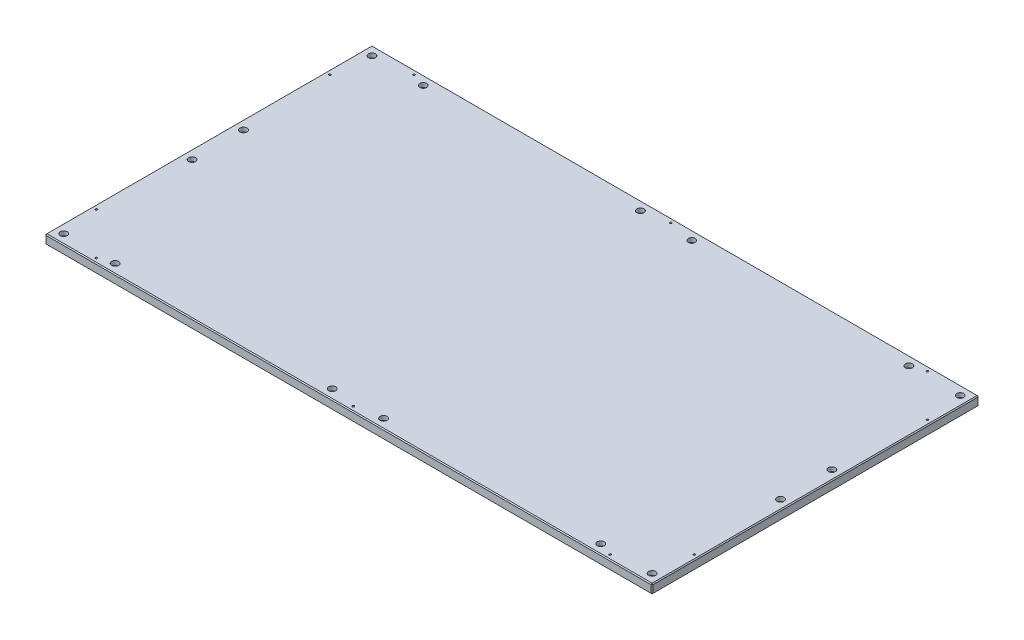
from build123d import *

# Parameters (mm, degrees)
SKETCH_1_W                          = 1300
SKETCH_1_H                          = 700
EXTRUDE_1_DEPTH                     = 10
CHAMFER_1_SIZE                      = 2
HOLE_WIZARD_1_D                     = 9
HOLE_WIZARD_1_CBORE_D               = 15
HOLE_WIZARD_1_CBORE_DEPTH           = 9
PATTERN_LINEAR_1_COUNT              = 2
PATTERN_LINEAR_1_PITCH              = 110
HOLE_WIZARD_2_D                     = 9
HOLE_WIZARD_2_CBORE_D               = 15
HOLE_WIZARD_2_CBORE_DEPTH           = 9
PATTERN_LINEAR_2_COUNT              = 2
PATTERN_LINEAR_2_PITCH              = 110
MIRROR_1_COPY_1_D                   = 9
MIRROR_1_COPY_1_CBORE_D             = 15
MIRROR_1_COPY_1_CBORE_DEPTH         = 9
MIRROR_2_COPY_1_D                   = 9
MIRROR_2_COPY_1_CBORE_D             = 15
MIRROR_2_COPY_1_CBORE_DEPTH         = 9
PATTERN_LINEAR_3_COUNT              = 3
PATTERN_LINEAR_3_PITCH              = 575
PATTERN_LINEAR_3_COPY_1_D           = 9
PATTERN_LINEAR_3_COPY_1_CBORE_D     = 15
PATTERN_LINEAR_3_COPY_1_CBORE_DEPTH = 9
PATTERN_LINEAR_3_COPY_2_D           = 9
PATTERN_LINEAR_3_COPY_2_CBORE_D     = 15
PATTERN_LINEAR_3_COPY_2_CBORE_DEPTH = 9
PATTERN_LINEAR_3_COPY_3_D           = 9
PATTERN_LINEAR_3_COPY_3_CBORE_D     = 15
PATTERN_LINEAR_3_COPY_3_CBORE_DEPTH = 9
PATTERN_LINEAR_3_COPY_4_D           = 9
PATTERN_LINEAR_3_COPY_4_CBORE_D     = 15
PATTERN_LINEAR_3_COPY_4_CBORE_DEPTH = 9
PATTERN_LINEAR_3_COPY_5_D           = 9
PATTERN_LINEAR_3_COPY_5_CBORE_D     = 15
PATTERN_LINEAR_3_COPY_5_CBORE_DEPTH = 9
PATTERN_LINEAR_3_COPY_6_D           = 9
PATTERN_LINEAR_3_COPY_6_CBORE_D     = 15
PATTERN_LINEAR_3_COPY_6_CBORE_DEPTH = 9
PATTERN_LINEAR_4_COUNT              = 3
PATTERN_LINEAR_4_PITCH              = 550


with BuildPart() as part:
    # 草图1 → 凸台-拉伸1 (new, symmetric)
    with BuildSketch(Plane(origin=(0, 0, 0), x_dir=(1, 0, 0), z_dir=(0, 1, 0))):
        Rectangle(SKETCH_1_W, SKETCH_1_H)
    extrude(amount=EXTRUDE_1_DEPTH, both=True)

    # 倒角1
    chamfer_1_edges = [part.edges().sort_by_distance(p)[0] for p in [
        (650, 10, 0),
        (0, 10, -350),
        (-650, 10, 0),
        (0, -10, -350),
        (650, -10, 0),
        (0, -10, 350),
        (-650, -10, 0),
        (0, 10, 350),
        (-650, 0, -350),
        (650, 0, -350),
        (650, 0, 350),
        (-650, 0, 350),
    ]]
    chamfer(chamfer_1_edges, length=CHAMFER_1_SIZE)

    # 打孔尺寸根据内六角圆柱头螺钉的类型1 (through all)
    with Locations(Plane(origin=(630, 10, -330), x_dir=(0, 0, 1), z_dir=(0, 1, 0))):
        with Locations((0, 0)):
            hole_wizard_1 = CounterBoreHole(HOLE_WIZARD_1_D / 2, HOLE_WIZARD_1_CBORE_D / 2, HOLE_WIZARD_1_CBORE_DEPTH)

    # 阵列(线性)1: 打孔尺寸根据内六角圆柱头螺钉的类型1 ×2
    with Locations(*[(-i * PATTERN_LINEAR_1_PITCH, 0, 0) for i in range(1, PATTERN_LINEAR_1_COUNT)]):
        add(hole_wizard_1, mode=Mode.SUBTRACT)

    # 打孔尺寸根据内六角圆柱头螺钉的类型2 (through all)
    with Locations(Plane(origin=(630, 10, -55), x_dir=(0, 0, 1), z_dir=(0, 1, 0))):
        with Locations((0, 0)):
            hole_wizard_2 = CounterBoreHole(HOLE_WIZARD_2_D / 2, HOLE_WIZARD_2_CBORE_D / 2, HOLE_WIZARD_2_CBORE_DEPTH)

    # 阵列(线性)2: 打孔尺寸根据内六角圆柱头螺钉的类型2 ×2
    with Locations(*[(0, 0, i * PATTERN_LINEAR_2_PITCH) for i in range(1, PATTERN_LINEAR_2_COUNT)]):
        add(hole_wizard_2, mode=Mode.SUBTRACT)

    # 镜向1: 打孔尺寸根据内六角圆柱头螺钉的类型2 across plane
    add(hole_wizard_2.mirror(Plane(origin=(0, 0, 0), x_dir=(0, 0, 1), z_dir=(1, 0, 0))), mode=Mode.SUBTRACT)

    # 镜向1 copy 1 (through all)
    with Locations(Plane(origin=(-630, 10, 55), x_dir=(0, 0, 1), z_dir=(0, 1, 0))):
        with Locations((0, 0)):
            CounterBoreHole(MIRROR_1_COPY_1_D / 2, MIRROR_1_COPY_1_CBORE_D / 2, MIRROR_1_COPY_1_CBORE_DEPTH)

    # 镜向2: 打孔尺寸根据内六角圆柱头螺钉的类型1 across plane
    add(hole_wizard_1.mirror(Plane.XY), mode=Mode.SUBTRACT)

    # 镜向2 copy 1 (through all)
    with Locations(Plane(origin=(520, 10, 330), x_dir=(0, 0, -1), z_dir=(0, 1, 0))):
        with Locations((0, 0)):
            CounterBoreHole(MIRROR_2_COPY_1_D / 2, MIRROR_2_COPY_1_CBORE_D / 2, MIRROR_2_COPY_1_CBORE_DEPTH)

    # 阵列(线性)3: 打孔尺寸根据内六角圆柱头螺钉的类型1 ×3
    with Locations(*[(-i * PATTERN_LINEAR_3_PITCH, 0, 0) for i in range(1, PATTERN_LINEAR_3_COUNT)]):
        add(hole_wizard_1, mode=Mode.SUBTRACT)

    # 阵列(线性)3 copy 1 (through all)
    with Locations(Plane(origin=(-55, 10, -330), x_dir=(0, 0, 1), z_dir=(0, 1, 0))):
        with Locations((0, 0)):
            CounterBoreHole(PATTERN_LINEAR_3_COPY_1_D / 2, PATTERN_LINEAR_3_COPY_1_CBORE_D / 2, PATTERN_LINEAR_3_COPY_1_CBORE_DEPTH)

    # 阵列(线性)3 copy 2 (through all)
    with Locations(Plane(origin=(-630, 10, -330), x_dir=(0, 0, 1), z_dir=(0, 1, 0))):
        with Locations((0, 0)):
            CounterBoreHole(PATTERN_LINEAR_3_COPY_2_D / 2, PATTERN_LINEAR_3_COPY_2_CBORE_D / 2, PATTERN_LINEAR_3_COPY_2_CBORE_DEPTH)

    # 阵列(线性)3 copy 3 (through all)
    with Locations(Plane(origin=(55, 10, 330), x_dir=(0, 0, -1), z_dir=(0, 1, 0))):
        with Locations((0, 0)):
            CounterBoreHole(PATTERN_LINEAR_3_COPY_3_D / 2, PATTERN_LINEAR_3_COPY_3_CBORE_D / 2, PATTERN_LINEAR_3_COPY_3_CBORE_DEPTH)

    # 阵列(线性)3 copy 4 (through all)
    with Locations(Plane(origin=(-520, 10, 330), x_dir=(0, 0, -1), z_dir=(0, 1, 0))):
        with Locations((0, 0)):
            CounterBoreHole(PATTERN_LINEAR_3_COPY_4_D / 2, PATTERN_LINEAR_3_COPY_4_CBORE_D / 2, PATTERN_LINEAR_3_COPY_4_CBORE_DEPTH)

    # 阵列(线性)3 copy 5 (through all)
    with Locations(Plane(origin=(-55, 10, 330), x_dir=(0, 0, -1), z_dir=(0, 1, 0))):
        with Locations((0, 0)):
            CounterBoreHole(PATTERN_LINEAR_3_COPY_5_D / 2, PATTERN_LINEAR_3_COPY_5_CBORE_D / 2, PATTERN_LINEAR_3_COPY_5_CBORE_DEPTH)

    # 阵列(线性)3 copy 6 (through all)
    with Locations(Plane(origin=(-630, 10, 330), x_dir=(0, 0, -1), z_dir=(0, 1, 0))):
        with Locations((0, 0)):
            CounterBoreHole(PATTERN_LINEAR_3_COPY_6_D / 2, PATTERN_LINEAR_3_COPY_6_CBORE_D / 2, PATTERN_LINEAR_3_COPY_6_CBORE_DEPTH)

    # 草图14 → M5 螺纹孔1 (revolve, cut)
    with BuildSketch(Plane(origin=(550, 10, -340), x_dir=(0, 0, 1), z_dir=(1, 0, 0))):
        Polygon((0, 0), (0, 23.6618073), (2.1, 22.4), (2.1, 0), align=None)
    hole_wizard_m5_1 = revolve(axis=Axis((550, 16.35, -340), (0, -1, 0)), mode=Mode.SUBTRACT)

    # 阵列(线性)4: M5 螺纹孔1 ×3
    with Locations(*[(-i * PATTERN_LINEAR_4_PITCH, 0, 0) for i in range(1, PATTERN_LINEAR_4_COUNT)]):
        add(hole_wizard_m5_1, mode=Mode.SUBTRACT)

    # 镜向3: M5 螺纹孔1 across plane
    add(hole_wizard_m5_1.mirror(Plane.XY), mode=Mode.SUBTRACT)

    # 镜向3 copy 1 sketch → 镜向3 copy 1 (revolve, cut)
    with BuildSketch(Plane(origin=(0, 10, 340), x_dir=(0, 0, -1), z_dir=(1, 0, 0))):
        Polygon((0, 0), (0, -23.6618073), (2.1, -22.4), (2.1, 0), align=None)
    revolve(axis=Axis((0, 16.35, 340), (0, 1, 0)), mode=Mode.SUBTRACT)

    # 镜向3 copy 2 sketch → 镜向3 copy 2 (revolve, cut)
    with BuildSketch(Plane(origin=(-550, 10, 340), x_dir=(0, 0, -1), z_dir=(1, 0, 0))):
        Polygon((0, 0), (0, -23.6618073), (2.1, -22.4), (2.1, 0), align=None)
    revolve(axis=Axis((-550, 16.35, 340), (0, 1, 0)), mode=Mode.SUBTRACT)

    # 草图15 → M5 螺纹孔2 (revolve, cut)
    with BuildSketch(Plane(origin=(-640, 10, -250), x_dir=(0, 0, 1), z_dir=(1, 0, 0))):
        Polygon((0, 0), (0, 23.6618073), (2.1, 22.4), (2.1, 0), align=None)
    hole_wizard_m5_2 = revolve(axis=Axis((-640, 16.35, -250), (0, -1, 0)), mode=Mode.SUBTRACT)

    # 镜向4: M5 螺纹孔2 across plane
    add(hole_wizard_m5_2.mirror(Plane.XY), mode=Mode.SUBTRACT)

    # 镜向5: M5 螺纹孔2 across plane
    add(hole_wizard_m5_2.mirror(Plane(origin=(0, 0, 0), x_dir=(0, 0, 1), z_dir=(1, 0, 0))), mode=Mode.SUBTRACT)

    # 镜向5 copy 1 sketch → 镜向5 copy 1 (revolve, cut)
    with BuildSketch(Plane(origin=(640, 10, 250), x_dir=(0, 0, -1), z_dir=(-1, 0, 0))):
        Polygon((0, 0), (0, 23.6618073), (2.1, 22.4), (2.1, 0), align=None)
    revolve(axis=Axis((640, 16.35, 250), (0, -1, 0)), mode=Mode.SUBTRACT)


solid = part.part
